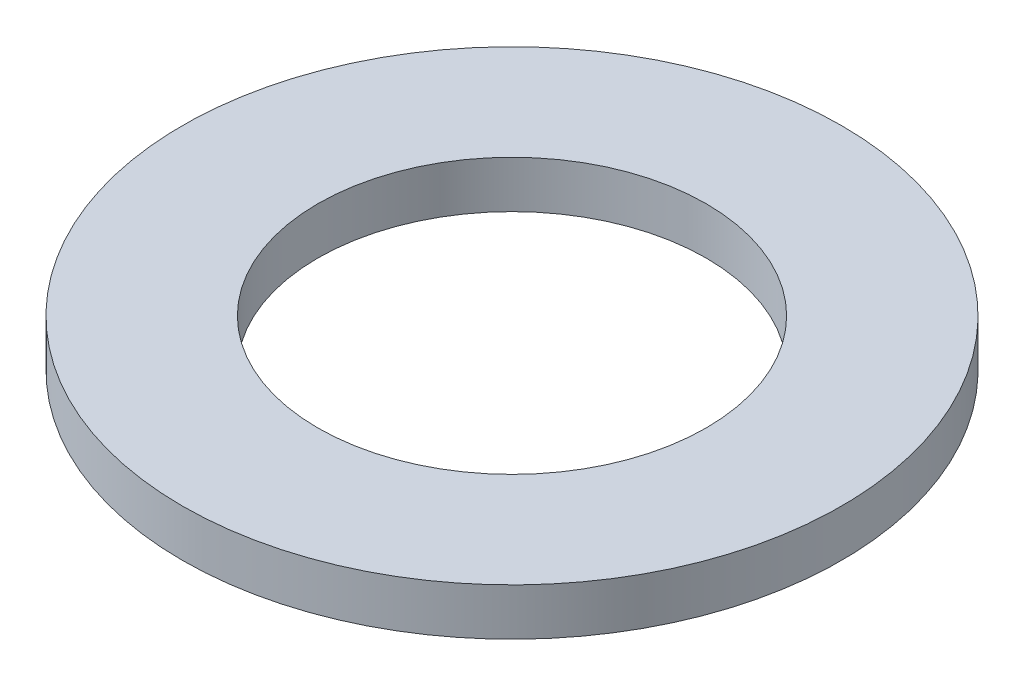
from build123d import *

# Parameters (mm, degrees)
SKETCH1_W = 11.5
SKETCH1_H = 4


with BuildPart() as part:
    # Sketch1 → Base-Revolve (revolve)
    with BuildSketch(Plane.XY, mode=Mode.PRIVATE) as base_revolve_sk:
        with Locations((-22.25, 10.644507042)):
            Rectangle(SKETCH1_W, SKETCH1_H)
    revolve(base_revolve_sk.sketch.rotate(Axis((0, 0, 0), (0, 1, 0)), 270), axis=Axis((0, 0, 0), (0, 1, 0)))


solid = part.part
